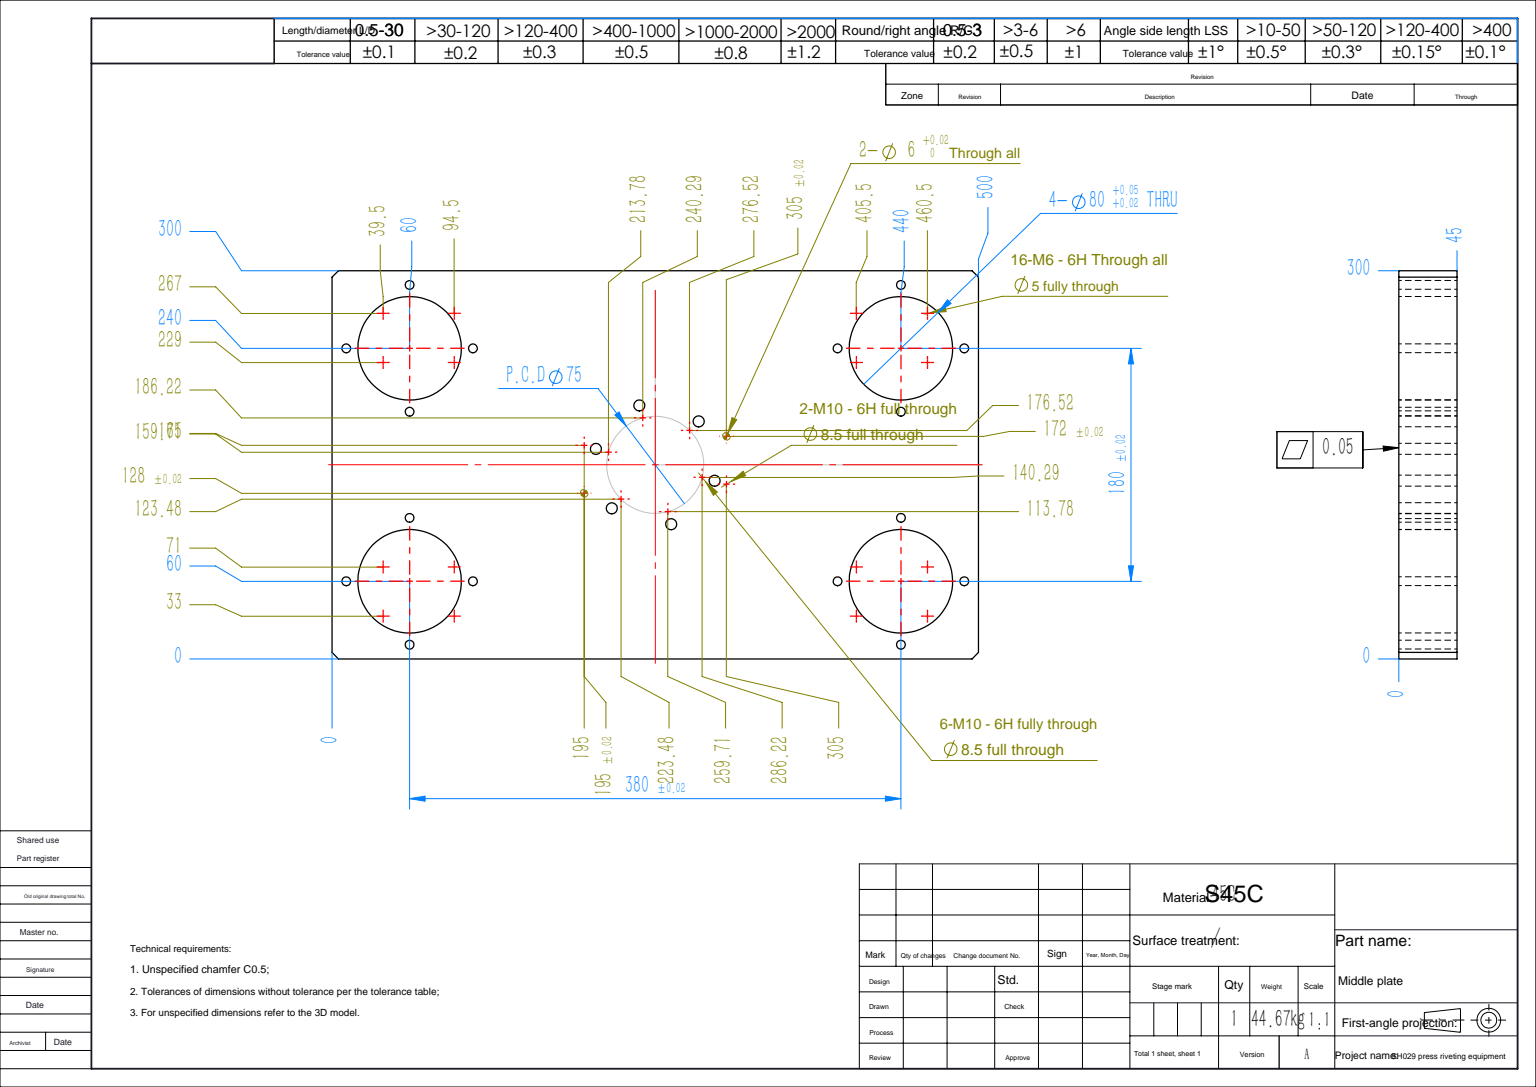
SolidWorks part; units mm, degrees
material "S45C"
ref_plane "前视" through (0, 0, 0) normal (0, 0, 1) x (1, 0, 0)
ref_plane "上视" through (0, 0, 0) normal (0, 1, 0) x (1, 0, 0)
ref_plane "右视" through (0, 0, 0) normal (1, 0, 0) x (0, 0, -1)
sketch "草图1" plane through (0, 0, 0) normal (0, 1, 0) x (1, 0, 0)
  line L1 (-250, 150) -> (250, 150)
  line L2 (-250, 150) -> (-250, -150)
  line L3 (-250, -150) -> (250, -150)
  line L4 (250, 150) -> (250, -150)
  line L5 (-250, 150) -> (250, -150) construction
  line L6 (-250, -150) -> (250, 150) construction
  point P0 (0, 0)
  dimension "D1" = 500
  dimension "D2" = 300
extrude "凸台-拉伸1" add sketch "草图1" along normal blind 45
chamfer "倒角1" distance 5 angle 45 4 edges at (-250, 22.5, -150) (-250, 22.5, 150) (250, 22.5, -150) (250, 22.5, 150)
sketch "草图6" plane through (0, 45, 0) normal (0, 1, 0) x (1, 0, 0)
  circle A0 centre (190, -90) radius 40
  circle A1 centre (190, 90) radius 40
  circle A2 centre (-190, 90) radius 40
  circle A3 centre (-190, -90) radius 40
  dimension "D1" = 80
extrude "切除-拉伸1" cut sketch "草图6" against normal through all
hole_wizard "M10 螺纹孔3" positions "草图14" profile "草图13" tap size "M10" standard "GB" end condition through all
sketch "草图14" plane through (0, 45, 0) normal (0, 1, 0) x (1, 0, 0)
  circle A0 centre (-12.2939, 45.8815) radius 5.5 construction
  circle A1 centre (-45.8815, 12.2939) radius 5.5 construction
  circle A2 centre (-33.5876, -33.5876) radius 5.5 construction
  circle A3 centre (12.2939, -45.8815) radius 5.5 construction
  circle A4 centre (45.8815, -12.2939) radius 5.5 construction
  circle A5 centre (33.5876, 33.5876) radius 5.5 construction
  point P1 (-12.2939, 45.8815)
  point P5 (-45.8815, 12.2939)
  point P9 (-33.5876, -33.5876)
  point P13 (12.2939, -45.8815)
  point P17 (45.8815, -12.2939)
  point P21 (33.5876, 33.5876)
sketch "草图13" plane through (-12.2939, 45, -45.8815) normal (1, 0, 0) x (0, 0, 1)
  line L0 (0, 0) -> (0, 45)
  line L1 (0, 45) -> (4.25, 45)
  line L2 (4.25, 45) -> (4.25, 0)
  line L5 (4.25, 0) -> (0, 0)
  line L11 (0, -6.35) -> (0, 107.95) construction
  dimension "通孔螺纹孔钻头直径" = 8.5
  dimension "通孔螺纹孔钻头深度" = 45
cosmetic thread "孔螺纹线1" parameters "D2"=10
cosmetic thread "孔螺纹线2" parameters "D2"=10
cosmetic thread "孔螺纹线3" parameters "D2"=10
cosmetic thread "孔螺纹线4" parameters "D2"=10
cosmetic thread "孔螺纹线5" parameters "D2"=10
cosmetic thread "孔螺纹线6" parameters "D2"=10
hole_wizard "M8 螺纹孔1" positions "草图16" profile "草图15" tap size "M8" standard "GB" end condition through all
sketch "草图16" plane through (0, 45, 0) normal (0, 1, 0) x (1, 0, 0)
  circle A0 centre (239, -90) radius 4.5 construction
  circle A1 centre (190, -139) radius 4.5 construction
  circle A2 centre (141, -90) radius 4.5 construction
  circle A3 centre (190, -41) radius 4.5 construction
  circle A4 centre (239, 90) radius 4.5 construction
  circle A5 centre (190, 41) radius 4.5 construction
  circle A6 centre (141, 90) radius 4.5 construction
  circle A7 centre (190, 139) radius 4.5 construction
  circle A8 centre (-141, -90) radius 4.5 construction
  circle A9 centre (-190, -139) radius 4.5 construction
  circle A10 centre (-239, -90) radius 4.5 construction
  circle A11 centre (-190, -41) radius 4.5 construction
  circle A12 centre (-141, 90) radius 4.5 construction
  circle A13 centre (-190, 41) radius 4.5 construction
  circle A14 centre (-239, 90) radius 4.5 construction
  circle A15 centre (-190, 139) radius 4.5 construction
  point P1 (239, -90)
  point P5 (190, -139)
  point P9 (141, -90)
  point P13 (190, -41)
  point P17 (239, 90)
  point P21 (190, 41)
  point P25 (141, 90)
  point P29 (190, 139)
  point P33 (-141, -90)
  point P37 (-190, -139)
  point P41 (-239, -90)
  point P45 (-190, -41)
  point P49 (-141, 90)
  point P53 (-190, 41)
  point P57 (-239, 90)
  point P61 (-190, 139)
sketch "草图15" plane through (239, 45, 90) normal (1, 0, 0) x (0, 0, 1)
  line L0 (0, 0) -> (0, 45)
  line L1 (0, 45) -> (3.4, 45)
  line L2 (3.4, 45) -> (3.4, 0)
  line L5 (3.4, 0) -> (0, 0)
  line L11 (0, -6.35) -> (0, 107.95) construction
  dimension "通孔螺纹孔钻头直径" = 6.8
  dimension "通孔螺纹孔钻头深度" = 45
cosmetic thread "孔螺纹线7" parameters "D2"=8
cosmetic thread "孔螺纹线8" parameters "D2"=8
cosmetic thread "孔螺纹线9" parameters "D2"=8
cosmetic thread "孔螺纹线10" parameters "D2"=8
cosmetic thread "孔螺纹线11" parameters "D2"=8
cosmetic thread "孔螺纹线12" parameters "D2"=8
cosmetic thread "孔螺纹线13" parameters "D2"=8
cosmetic thread "孔螺纹线14" parameters "D2"=8
cosmetic thread "孔螺纹线15" parameters "D2"=8
cosmetic thread "孔螺纹线16" parameters "D2"=8
cosmetic thread "孔螺纹线17" parameters "D2"=8
cosmetic thread "孔螺纹线18" parameters "D2"=8
cosmetic thread "孔螺纹线19" parameters "D2"=8
cosmetic thread "孔螺纹线20" parameters "D2"=8
cosmetic thread "孔螺纹线21" parameters "D2"=8
cosmetic thread "孔螺纹线22" parameters "D2"=8
